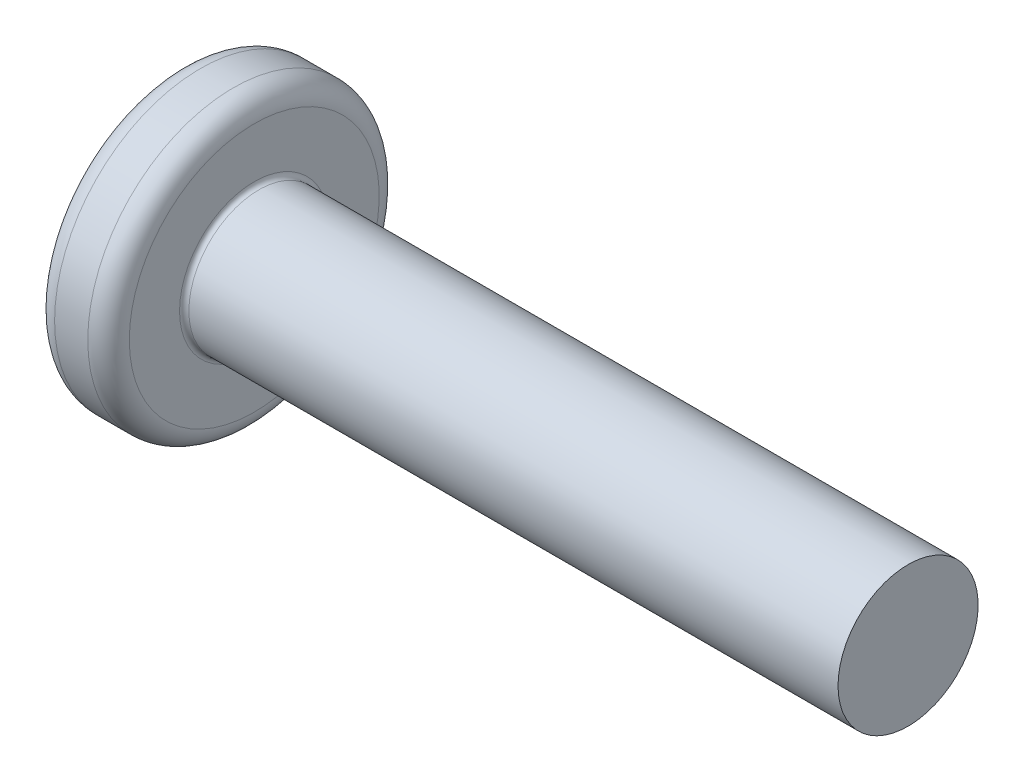
SolidWorks part; units mm, degrees
ref_plane "Front Plane" through (0, 0, 0) normal (0, 0, 1) x (1, 0, 0)
ref_plane "Top Plane" through (0, 0, 0) normal (0, 1, 0) x (1, 0, 0)
ref_plane "Right Plane" through (0, 0, 0) normal (1, 0, 0) x (0, 0, -1)
sketch "Dimensioned Sketch" plane through (0, 0, 0) normal (0, 0, 1) x (1, 0, 0)
  line L0 (0, 0) -> (15.6, 0) construction
  line L1 (0, 0) -> (0, 2.6752)
  line L2 (0.4448, 3.12) -> (1.1552, 3.12)
  line L3 (1.6, 2.6752) -> (1.6, 1.6)
  line L4 (1.7, 1.5) -> (15.6, 1.5)
  line L5 (15.6, 1.5) -> (15.6, 0)
  line L6 (0, 0) -> (15.6, 0)
  arc A0 (1.1552, 3.12) -> (1.6, 2.6752) centre (1.1552, 2.6752) cw
  arc A1 (0, 2.6752) -> (0.4448, 3.12) centre (0.4448, 2.6752) cw
  arc A2 (1.6, 1.6) -> (1.7, 1.5) centre (1.7, 1.6) ccw
  point P9 (1.6, 3.12)
  point P12 (0, 3.12)
  point P15 (1.6, 1.5)
  dimension "D1" = 0.4448
  dimension "r" = 0.1
  dimension "dk" = 6.24
  dimension "k" = 1.6
  dimension "l" = 14
  dimension "d" = 3
revolve "Revolve3" add sketch "Dimensioned Sketch" angle 360 about L0
